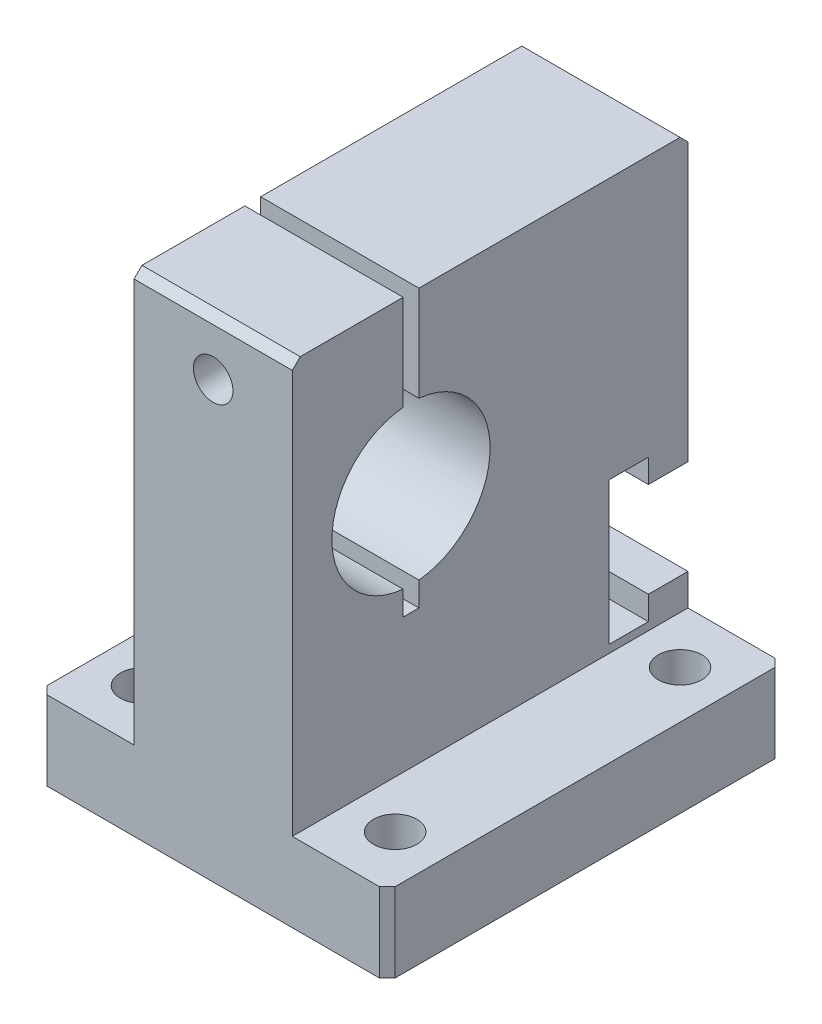
from build123d import *

# Parameters (mm, degrees)
BOSS_EXTRUDE1_DEPTH                                  = 50
CUT_EXTRUDE1_REACH                                   = 92.995
SKETCH2_R                                            = 2.75
CUT_EXTRUDE2_REACH                                   = 87.837
HOLE_SIZE_PER_SOCKET_HEAD_CAP_SCREW_TYPE_D           = 6.6
HOLE_SIZE_PER_SOCKET_HEAD_CAP_SCREW_TYPE_DEPTH       = 34
HOLE_SIZE_PER_SOCKET_HEAD_CAP_SCREW_TYPE_CBORE_D     = 11
HOLE_SIZE_PER_SOCKET_HEAD_CAP_SCREW_TYPE_CBORE_DEPTH = 6.8
M6_TAPPED_HOLE1_D                                    = 5
CHAMFER1_SIZE                                        = 1


with BuildPart() as part:
    # Sketch1 → Boss-Extrude1 (new body)
    with BuildSketch(Plane.XY):
        Polygon((32, 10), (44, 10), (44, 0), (0, 0), (0, 10), (12, 10), (12, 62), (32, 62), align=None)
    extrude(amount=BOSS_EXTRUDE1_DEPTH)

    # Sketch2 → Cut-Extrude1 (cut, up to next)
    with BuildSketch(Plane.XZ, mode=Mode.PRIVATE) as cut_extrude1_sk1:
        with Locations(Location((6, 43, 0), (0, 0, 270))):
            Circle(SKETCH2_R)
    cut_extrude1_tool1 = extrude(cut_extrude1_sk1.sketch, amount=-CUT_EXTRUDE1_REACH, mode=Mode.PRIVATE) & part.part
    # Sketch2 → Cut-Extrude1 (cut, up to next)
    with BuildSketch(Plane.XZ, mode=Mode.PRIVATE) as cut_extrude1_sk2:
        with Locations(Location((6, 7, 0), (0, 0, 270))):
            Circle(SKETCH2_R)
    cut_extrude1_tool2 = extrude(cut_extrude1_sk2.sketch, amount=-CUT_EXTRUDE1_REACH, mode=Mode.PRIVATE) & part.part
    # Sketch2 → Cut-Extrude1 (cut, up to next)
    with BuildSketch(Plane.XZ, mode=Mode.PRIVATE) as cut_extrude1_sk3:
        with Locations(Location((38, 43, 0), (0, 0, 270))):
            Circle(SKETCH2_R)
    cut_extrude1_tool3 = extrude(cut_extrude1_sk3.sketch, amount=-CUT_EXTRUDE1_REACH, mode=Mode.PRIVATE) & part.part
    # Sketch2 → Cut-Extrude1 (cut, up to next)
    with BuildSketch(Plane.XZ, mode=Mode.PRIVATE) as cut_extrude1_sk4:
        with Locations(Location((38, 7, 0), (0, 0, 270))):
            Circle(SKETCH2_R)
    cut_extrude1_tool4 = extrude(cut_extrude1_sk4.sketch, amount=-CUT_EXTRUDE1_REACH, mode=Mode.PRIVATE) & part.part
    add(cut_extrude1_tool1.solids().sort_by_distance((6, 0, 43))[0], mode=Mode.SUBTRACT)
    add(cut_extrude1_tool2.solids().sort_by_distance((6, 0, 7))[0], mode=Mode.SUBTRACT)
    add(cut_extrude1_tool3.solids().sort_by_distance((38, 0, 43))[0], mode=Mode.SUBTRACT)
    add(cut_extrude1_tool4.solids().sort_by_distance((38, 0, 7))[0], mode=Mode.SUBTRACT)

    # Sketch3 → Cut-Extrude2 (cut, up to next)
    with BuildSketch(Plane.ZY.offset(-12), mode=Mode.PRIVATE) as cut_extrude2_sk1:
        with BuildLine():
            Line((34, 49.949874371), (34, 62))
            Line((34, 62), (36, 62))
            Line((36, 62), (36, 49.949874371))
            ThreePointArc((36, 49.949874371), (45, 40), (36, 30.050125629))
            Line((36, 30.050125629), (36, 27))
            Line((36, 27), (34, 27))
            Line((34, 27), (34, 30.050125629))
            ThreePointArc((34, 30.050125629), (25, 40), (34, 49.949874371))
        make_face()
    cut_extrude2_tool1 = extrude(cut_extrude2_sk1.sketch, amount=-CUT_EXTRUDE2_REACH, mode=Mode.PRIVATE) & part.part
    # Sketch3 → Cut-Extrude2 (cut, up to next)
    with BuildSketch(Plane.ZY.offset(-12), mode=Mode.PRIVATE) as cut_extrude2_sk2:
        Polygon((5, 26), (5, 29), (10, 29), (10, 11), (5, 11), (5, 14), (0, 14), (0, 26), align=None)
    cut_extrude2_tool2 = extrude(cut_extrude2_sk2.sketch, amount=-CUT_EXTRUDE2_REACH, mode=Mode.PRIVATE) & part.part
    add(cut_extrude2_tool1.solids().sort_by_distance((12, 40.915096, 35))[0], mode=Mode.SUBTRACT)
    add(cut_extrude2_tool2.solids().sort_by_distance((12, 20, 5.5))[0], mode=Mode.SUBTRACT)

    # Hole size per socket head cap screw type 1
    with Locations(Plane(origin=(0, 0, 0), x_dir=(-1, 0, 0), z_dir=(0, 0, -1))):
        with Locations((-22, 55)):
            CounterBoreHole(HOLE_SIZE_PER_SOCKET_HEAD_CAP_SCREW_TYPE_D / 2, HOLE_SIZE_PER_SOCKET_HEAD_CAP_SCREW_TYPE_CBORE_D / 2, HOLE_SIZE_PER_SOCKET_HEAD_CAP_SCREW_TYPE_CBORE_DEPTH, depth=HOLE_SIZE_PER_SOCKET_HEAD_CAP_SCREW_TYPE_DEPTH)

    # M6 Tapped Hole1 (through all)
    with Locations(Plane(origin=(0, 0, 0), x_dir=(-1, 0, 0), z_dir=(0, 0, -1))):
        with Locations((-22, 55)):
            Hole(M6_TAPPED_HOLE1_D / 2)

    # Chamfer1
    chamfer1_edges = [part.edges().sort_by_distance(p)[0] for p in [
        (44, 5, 50),
        (0, 5, 0),
        (22, 62, 50),
        (0, 5, 50),
        (22, 62, 0),
        (44, 5, 0),
    ]]
    chamfer(chamfer1_edges, length=CHAMFER1_SIZE)


solid = part.part
